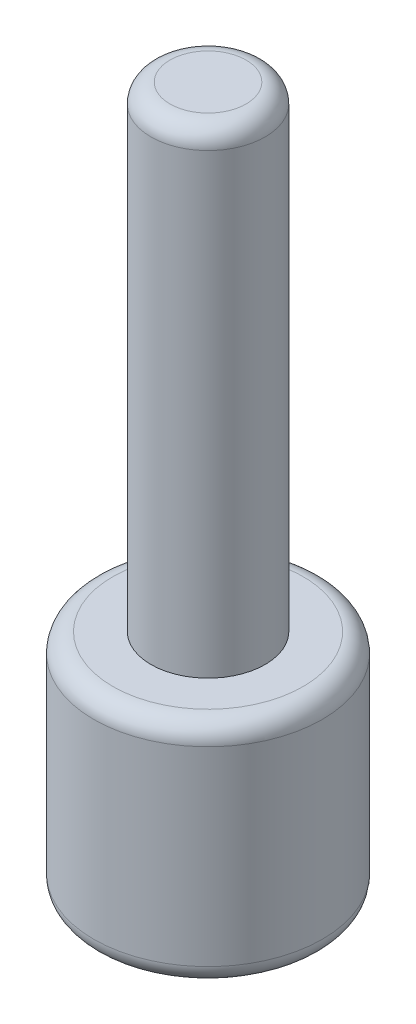
SolidWorks part; units mm, degrees
ref_plane "前视基准面" through (0, 0, 0) normal (0, 0, 1) x (1, 0, 0)
ref_plane "上视基准面" through (0, 0, 0) normal (0, 1, 0) x (1, 0, 0)
ref_plane "右视基准面" through (0, 0, 0) normal (1, 0, 0) x (0, 0, -1)
sketch "草图1" plane through (0, 0, 0) normal (0, 1, 0) x (1, 0, 0)
  circle A0 centre (0, 0) radius 6
extrude "凸台-拉伸1" add sketch "草图1" along normal blind 12
sketch "草图2" plane through (0, 12, 0) normal (0, 1, 0) x (1, 0, 0)
  circle A0 centre (0, 0) radius 3
extrude "凸台-拉伸2" add sketch "草图2" along normal blind 25
cosmetic thread "装饰螺纹线1" parameters "D2"=5
fillet "圆角1" radius 1 3 edges at (0, 0, 6) (0, 37, 3) (0, 12, 6)
